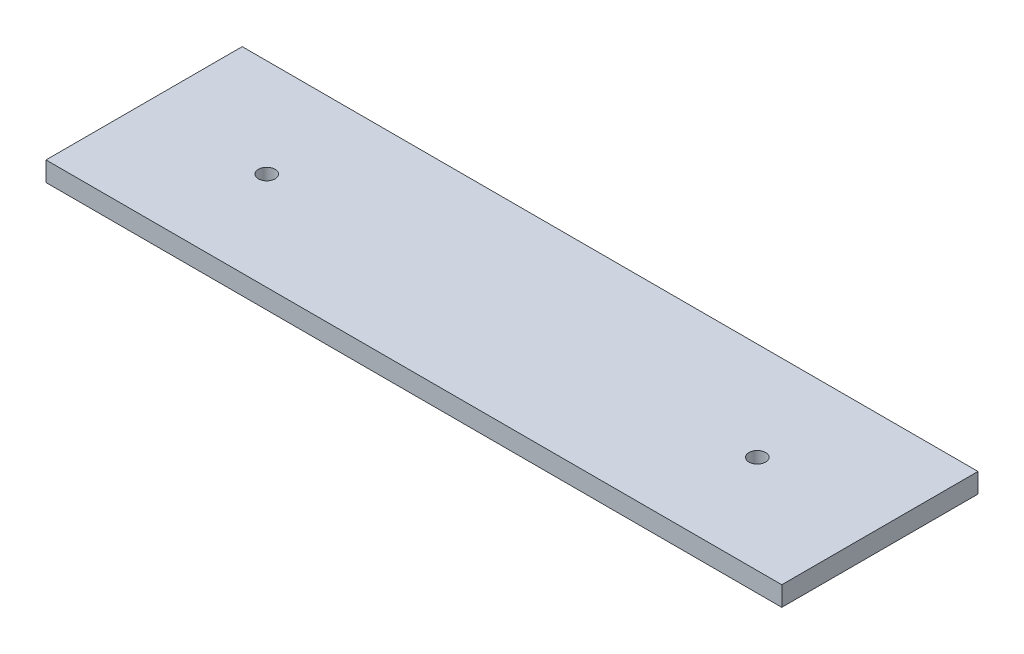
from build123d import *

# Parameters (mm, degrees)
SKETCH1_W           = 300
SKETCH1_H           = 80
BOSS_EXTRUDE1_DEPTH = 8
M8_TAPPED_HOLE1_D   = 6.8


with BuildPart() as part:
    # Sketch1 → Boss-Extrude1 (new body)
    with BuildSketch(Plane(origin=(0, 0, 0), x_dir=(1, 0, 0), z_dir=(0, 1, 0))):
        with Locations((150, 40)):
            Rectangle(SKETCH1_W, SKETCH1_H)
    extrude(amount=BOSS_EXTRUDE1_DEPTH)

    # M8 Tapped Hole1 (through all)
    with Locations(Plane(origin=(0, 8, 0), x_dir=(1, 0, 0), z_dir=(0, 1, 0))):
        with Locations((50, 40), (250, 40)):
            Hole(M8_TAPPED_HOLE1_D / 2)


solid = part.part
